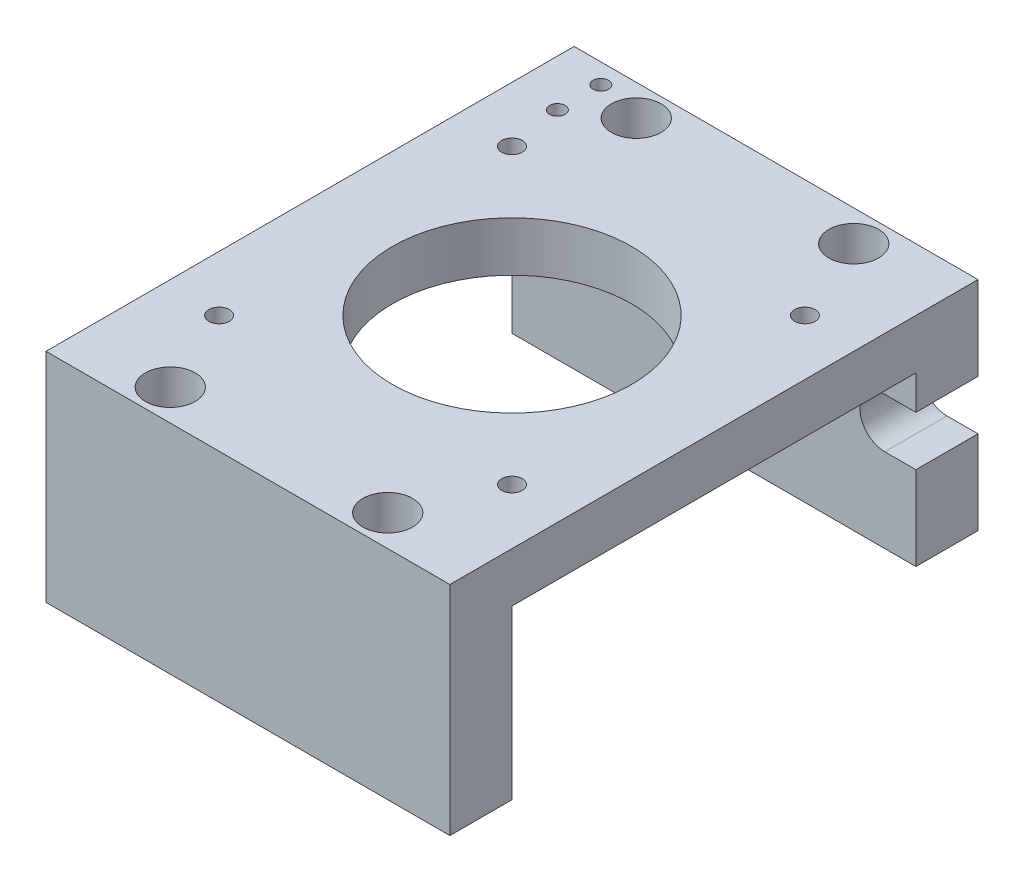
from build123d import *

# Parameters (mm, degrees)
SKETCH_1_W                = 65
SKETCH_1_H                = 85
EXTRUDE_1_DEPTH           = 35
SKETCH_2_W                = 109.971307268
SKETCH_2_H                = 65
CUT_EXTRUDE_1_DEPTH       = 27
SKETCH_3_R                = 19.25
CUT_EXTRUDE_2_DEPTH       = 64.933559263
HOLE_WIZARD_M4_1_D        = 3.3
HOLE_WIZARD_M3_1_D        = 2.5
HOLE_WIZARD_M3_1_DEPTH    = 12.5
HOLE_WIZARD_M3_1_TIP      = 0.751075774
CUT_EXTRUDE_3_DEPTH       = 15
HOLE_WIZARD_1_D           = 4.5
HOLE_WIZARD_1_CBORE_D     = 8
HOLE_WIZARD_1_CBORE_DEPTH = 20
HOLE_WIZARD_M3_3_D        = 2.5
HOLE_WIZARD_M3_3_DEPTH    = 9.5
HOLE_WIZARD_M3_3_TIP      = 0.751075774


with BuildPart() as part:
    # 草图1 → 凸台-拉伸1 (new body)
    with BuildSketch(Plane(origin=(0, 0, 0), x_dir=(1, 0, 0), z_dir=(0, 1, 0))):
        Rectangle(SKETCH_1_W, SKETCH_1_H)
    extrude(amount=EXTRUDE_1_DEPTH)

    # 草图2 → 切除-拉伸1 (cut)
    with BuildSketch(Plane.XZ):
        Rectangle(SKETCH_2_W, SKETCH_2_H)
    extrude(amount=-CUT_EXTRUDE_1_DEPTH, mode=Mode.SUBTRACT)

    # 草图3 → 切除-拉伸2 (cut, through all)
    with BuildSketch(Plane(origin=(0, 35, 0), x_dir=(1, 0, 0), z_dir=(0, 1, 0))):
        with Locations(Location((0, 0, 0), (0, 0, 270))):
            Circle(SKETCH_3_R)
    extrude(amount=-CUT_EXTRUDE_2_DEPTH, mode=Mode.SUBTRACT)

    # M4 螺纹孔1 (through all)
    with Locations(Plane(origin=(0, 35, 0), x_dir=(1, 0, 0), z_dir=(0, 1, 0))):
        with Locations((-23.57, 23.57), (23.57, 23.57), (-23.57, -23.57), (23.57, -23.57)):
            Hole(HOLE_WIZARD_M4_1_D / 2)

    # M3 螺纹孔1
    with Locations(Plane.ZY.offset(32.5)):
        with Locations((7.5, 31), (-7.5, 31)):
            Hole(HOLE_WIZARD_M3_1_D / 2, depth=HOLE_WIZARD_M3_1_DEPTH)
            with Locations((0, 0, -(HOLE_WIZARD_M3_1_DEPTH + HOLE_WIZARD_M3_1_TIP / 2))):  # 118° drill point
                Cone(0, HOLE_WIZARD_M3_1_D / 2, HOLE_WIZARD_M3_1_TIP, mode=Mode.SUBTRACT)

    # 草图10 → 切除-拉伸3 (cut)
    with BuildSketch(Plane(origin=(0, 0, -42.5), x_dir=(-1, 0, 0), z_dir=(0, 0, -1))):
        with BuildLine():
            Line((-27.5, 13.5), (-37.5, 13.5))
            ThreePointArc((-37.5, 13.5), (-41.5, 17.5), (-37.5, 21.5))
            Line((-37.5, 21.5), (-27.5, 21.5))
            ThreePointArc((-27.5, 21.5), (-23.5, 17.5), (-27.5, 13.5))
        make_face()
    extrude(amount=-CUT_EXTRUDE_3_DEPTH, mode=Mode.SUBTRACT)

    # 打孔尺寸(%根据)开槽圆柱头螺钉的类型1 (through all)
    with Locations(Plane(origin=(0, 35, 0), x_dir=(1, 0, 0), z_dir=(0, 1, 0))):
        with Locations((-17.5, 37.5), (17.5, 37.5), (-17.5, -37.5), (17.5, -37.5)):
            CounterBoreHole(HOLE_WIZARD_1_D / 2, HOLE_WIZARD_1_CBORE_D / 2, HOLE_WIZARD_1_CBORE_DEPTH)

    # M3 螺纹孔3
    with Locations(Plane(origin=(0, 35, 0), x_dir=(1, 0, 0), z_dir=(0, 1, 0))):
        with Locations((-24.99999811, 32.299994492), (-24.99999811, 39.299998272)):
            Hole(HOLE_WIZARD_M3_3_D / 2, depth=HOLE_WIZARD_M3_3_DEPTH)
            with Locations((0, 0, -(HOLE_WIZARD_M3_3_DEPTH + HOLE_WIZARD_M3_3_TIP / 2))):  # 118° drill point
                Cone(0, HOLE_WIZARD_M3_3_D / 2, HOLE_WIZARD_M3_3_TIP, mode=Mode.SUBTRACT)


solid = part.part
